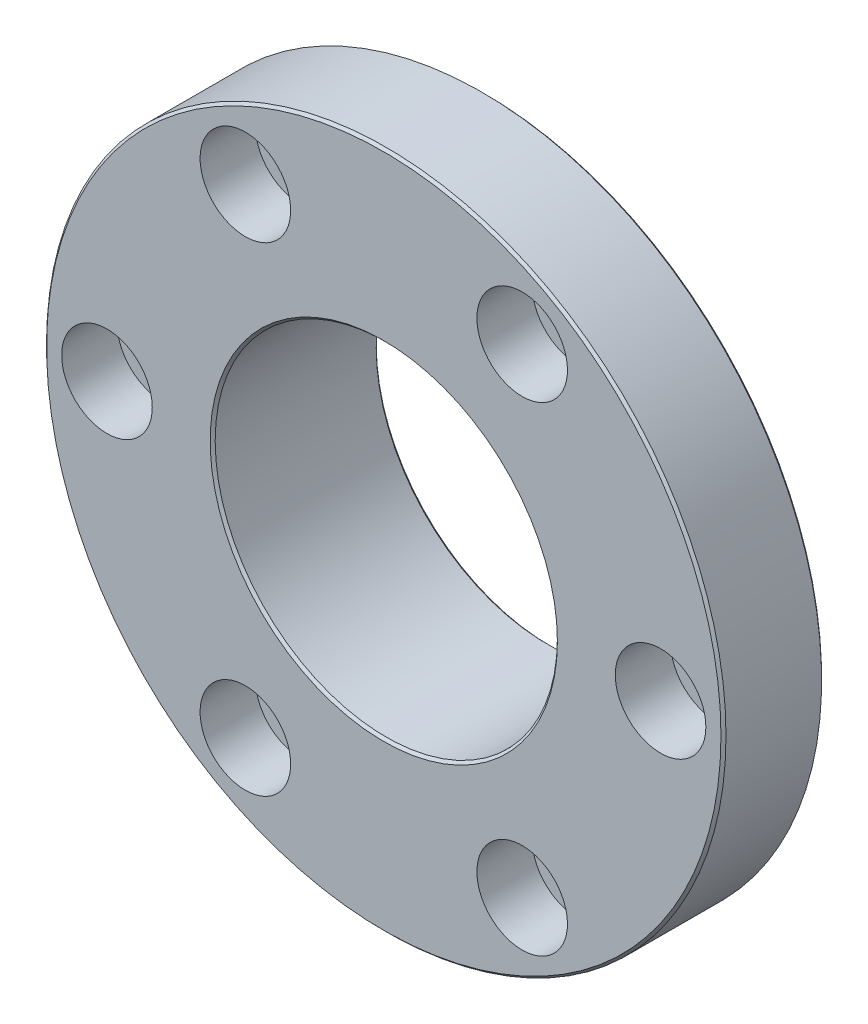
from build123d import *

# Parameters (mm, degrees)
HOLE_WIZARD_1_D           = 11
HOLE_WIZARD_1_CBORE_D     = 18
HOLE_WIZARD_1_CBORE_DEPTH = 11
PATTERN_CIRCULAR_1_COUNT  = 6
CHAMFER_1_SIZE            = 0.5


with BuildPart() as part:
    # 草图1 → 旋转1 (revolve)
    with BuildSketch(Plane(origin=(0, 0, 0), x_dir=(1, 0, 0), z_dir=(0, 1, 0))):
        Polygon((-34, 0), (-67.5, 0), (-67.5, 20), (-42.5, 20), (-42.5, 33), (-34, 33), align=None)
    revolve(axis=Axis((0, 0, 0), (0, 0, 1)))

    # 打孔尺寸(%根据)内六角圆柱头螺钉的类型1 (through all)
    with Locations(Plane.XY):
        with Locations((55, 0)):
            hole_wizard_1 = CounterBoreHole(HOLE_WIZARD_1_D / 2, HOLE_WIZARD_1_CBORE_D / 2, HOLE_WIZARD_1_CBORE_DEPTH)

    # 阵列(圆周)1: 打孔尺寸(%根据)内六角圆柱头螺钉的类型1 ×6 about axis
    pattern_circular_1_axis = Axis((0, 0, 0), (0, 0, 1))
    for i in range(1, PATTERN_CIRCULAR_1_COUNT):
        add(hole_wizard_1.rotate(pattern_circular_1_axis, i * 360 / PATTERN_CIRCULAR_1_COUNT), mode=Mode.SUBTRACT)

    # 倒角1
    chamfer_1_edges = [part.edges().sort_by_distance(p)[0] for p in [
        (67.5, 0, 0),
        (34, 0, 0),
        (34, 0, -33),
        (42.5, 0, -33),
        (67.5, 0, -20),
    ]]
    chamfer(chamfer_1_edges, length=CHAMFER_1_SIZE)


solid = part.part
